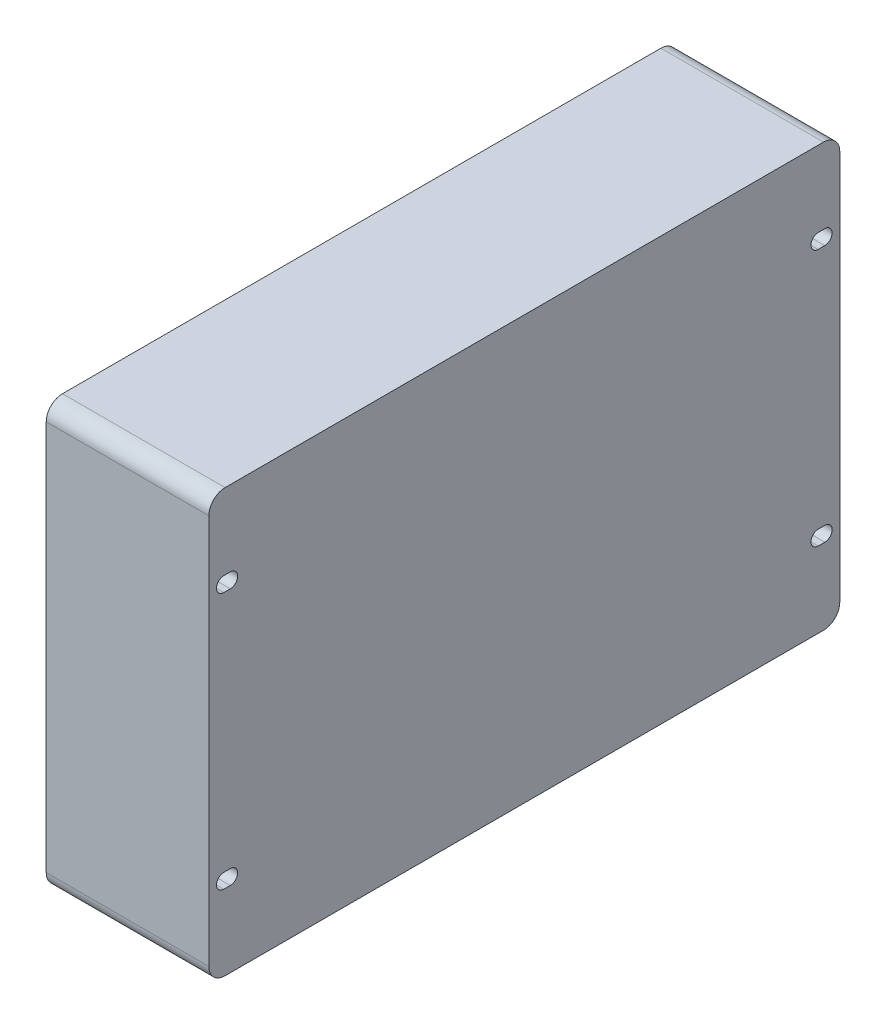
from build123d import *

# Parameters (mm, degrees)
SKETCH_1_W          = 388
SKETCH_1_H          = 260
EXTRUDE_1_DEPTH     = 50
CUT_EXTRUDE_1_DEPTH = 100
FILLET_1_R          = 10


with BuildPart() as part:
    # 草图1 → 凸台-拉伸1 (new, symmetric)
    with BuildSketch(Plane(origin=(0, 0, 0), x_dir=(0, 0, -1), z_dir=(1, 0, 0))):
        Rectangle(SKETCH_1_W, SKETCH_1_H)
    extrude(amount=EXTRUDE_1_DEPTH, both=True)

    # 草图2 → 切除-拉伸1 (cut)
    with BuildSketch(Plane(origin=(50, 0, 0), x_dir=(0, 0, -1), z_dir=(1, 0, 0))):
        with BuildLine():
            Line((-184.8, 83.5), (-180.8, 83.5))
            ThreePointArc((-180.8, 83.5), (-176.3, 79), (-180.8, 74.5))
            Line((-180.8, 74.5), (-184.8, 74.5))
            ThreePointArc((-184.8, 74.5), (-189.3, 79), (-184.8, 83.5))
        make_face()
        with BuildLine():
            Line((180.8, 83.5), (184.8, 83.5))
            ThreePointArc((184.8, 83.5), (189.3, 79), (184.8, 74.5))
            Line((184.8, 74.5), (180.8, 74.5))
            ThreePointArc((180.8, 74.5), (176.3, 79), (180.8, 83.5))
        make_face()
        with BuildLine():
            Line((180.8, -74.5), (184.8, -74.5))
            ThreePointArc((184.8, -74.5), (189.3, -79), (184.8, -83.5))
            Line((184.8, -83.5), (180.8, -83.5))
            ThreePointArc((180.8, -83.5), (176.3, -79), (180.8, -74.5))
        make_face()
        with BuildLine():
            Line((-184.8, -74.5), (-180.8, -74.5))
            ThreePointArc((-180.8, -74.5), (-176.3, -79), (-180.8, -83.5))
            Line((-180.8, -83.5), (-184.8, -83.5))
            ThreePointArc((-184.8, -83.5), (-189.3, -79), (-184.8, -74.5))
        make_face()
    extrude(amount=-CUT_EXTRUDE_1_DEPTH, mode=Mode.SUBTRACT)

    # 圆角1
    fillet_1_edges = [part.edges().sort_by_distance(p)[0] for p in [
        (0, 130, 194),
        (0, 130, -194),
        (0, -130, -194),
        (0, -130, 194),
    ]]
    fillet(fillet_1_edges, radius=FILLET_1_R)


solid = part.part
